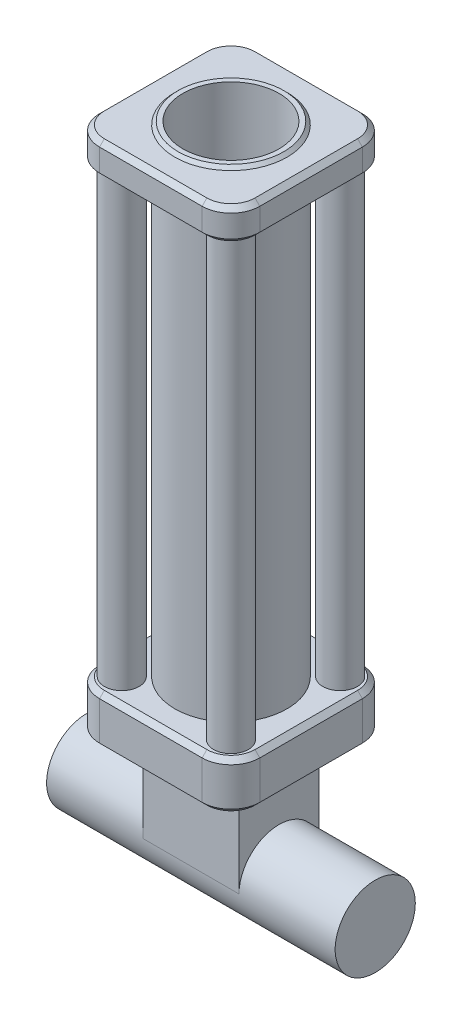
from build123d import *

# Parameters (mm, degrees)
SKETCH1_R                = 175
SKETCH1_R_2              = 150
BOSS_EXTRUDE1_DEPTH      = 1500
SKETCH2_W                = 500
SKETCH2_H                = 500
BOSS_EXTRUDE2_DEPTH      = 150
BOSS_EXTRUDE3_DEPTH      = 150
BOSS_EXTRUDE3_DEPTH_BACK = 150
BOSS_EXTRUDE4_DEPTH      = 450
BOSS_EXTRUDE4_DEPTH_BACK = 450
SKETCH4_R                = 125
CHAMFER2_SIZE            = 10
SKETCH5_W                = 500
SKETCH5_H                = 500
SKETCH5_R                = 154.887495166
BOSS_EXTRUDE5_DEPTH      = 100
BOSS_EXTRUDE6_REACH      = 1587.875
SKETCH6_R                = 54.226637303
CIRPATTERN1_COUNT        = 4
FILLET1_R                = 90
CHAMFER3_SIZE            = 15


with BuildPart() as part:
    # Sketch1 → Boss-Extrude1 (new body)
    with BuildSketch(Plane(origin=(0, 0, 0), x_dir=(1, 0, 0), z_dir=(0, 1, 0))):
        with Locations(Location((0, 0, 0), (0, 0, 270))):
            Circle(SKETCH1_R)
        with Locations(Location((0, 0, 0), (0, 0, 270))):
            Circle(SKETCH1_R_2, mode=Mode.SUBTRACT)
    extrude(amount=BOSS_EXTRUDE1_DEPTH)

    # Sketch2 → Boss-Extrude2 (add)
    with BuildSketch(Plane.XZ):
        Rectangle(SKETCH2_W, SKETCH2_H)
    extrude(amount=BOSS_EXTRUDE2_DEPTH)

    # Sketch3 → Boss-Extrude3 (add, two sides: drawn at the far end of the back side and taken through both)
    with BuildSketch(Plane(origin=(0, 0, 0), x_dir=(0, 0, -1), z_dir=(1, 0, 0)).offset(-BOSS_EXTRUDE3_DEPTH_BACK)):
        with BuildLine():
            Line((125, -150), (125, -450))
            ThreePointArc((125, -450), (0, -575), (-125, -450))
            Line((-125, -450), (-125, -150))
            Line((-125, -150), (125, -150))
        make_face()
    extrude(amount=BOSS_EXTRUDE3_DEPTH + BOSS_EXTRUDE3_DEPTH_BACK)

    # Sketch4 → Boss-Extrude4 (add, two sides: drawn at the far end of the back side and taken through both)
    with BuildSketch(Plane(origin=(0, 0, 0), x_dir=(0, 0, -1), z_dir=(1, 0, 0)).offset(-BOSS_EXTRUDE4_DEPTH_BACK)):
        with Locations((0, -450)):
            Circle(SKETCH4_R)
    extrude(amount=BOSS_EXTRUDE4_DEPTH + BOSS_EXTRUDE4_DEPTH_BACK)

    # Chamfer2
    chamfer2_edges = [part.edges().sort_by_distance(p)[0] for p in [
        (0, 1500, -175),
    ]]
    chamfer(chamfer2_edges, length=CHAMFER2_SIZE)

    # Sketch5 → Boss-Extrude5 (add)
    with BuildSketch(Plane(origin=(0, 1490, 0), x_dir=(1, 0, 0), z_dir=(0, 1, 0))):
        Rectangle(SKETCH5_W, SKETCH5_H)
        Circle(SKETCH5_R, mode=Mode.SUBTRACT)
    extrude(amount=-BOSS_EXTRUDE5_DEPTH)

    # Sketch6 → Boss-Extrude6 (add, up to next)
    with BuildSketch(Plane(origin=(0, 0, 0), x_dir=(1, 0, 0), z_dir=(0, 1, 0)), mode=Mode.PRIVATE) as boss_extrude6_sk1:
        with Locations(Location((-170.275340777, 170.275340777, 0), (0, 0, 90))):
            Circle(SKETCH6_R)
    boss_extrude6_tool1 = extrude(boss_extrude6_sk1.sketch, amount=BOSS_EXTRUDE6_REACH, mode=Mode.PRIVATE) - part.part
    boss_extrude6 = boss_extrude6_tool1.solids().sort_by_distance((-170.275341, 0, -170.275341))[0]
    add(boss_extrude6)

    # CirPattern1: Boss-Extrude6 ×4 about axis
    cirpattern1_axis = Axis((0, 0, 0), (0, 1, 0))
    for i in range(1, CIRPATTERN1_COUNT):
        add(boss_extrude6.rotate(cirpattern1_axis, i * 360 / CIRPATTERN1_COUNT))

    # Fillet1
    fillet1_edges = [part.edges().sort_by_distance(p)[0] for p in [
        (250, -75, -250),
        (250, -75, 250),
        (-250, -75, 250),
        (-250, -75, -250),
        (250, 1440, -250),
        (250, 1440, 250),
        (-250, 1440, 250),
        (-250, 1440, -250),
    ]]
    fillet(fillet1_edges, radius=FILLET1_R)

    # Chamfer3
    chamfer3_edges = [part.edges().sort_by_distance(p)[0] for p in [
        (250, -150, 0),
        (0, 0, -250),
        (-250, 0, 0),
        (0, 0, 250),
        (-223.639610307, 0, -223.639610307),
        (-223.639610307, 0, 223.639610307),
        (223.639610307, 0, 223.639610307),
        (223.639610307, 0, -223.639610307),
        (0, -150, -250),
        (0, -150, 250),
        (-250, -150, 0),
        (-223.639610307, -150, -223.639610307),
        (-223.639610307, -150, 223.639610307),
        (223.639610307, -150, 223.639610307),
        (223.639610307, -150, -223.639610307),
        (0, 1490, -250),
        (0, 1390, -250),
        (250, 1490, 0),
        (-250, 1490, 0),
        (0, 1490, 250),
        (223.639610307, 1490, -223.639610307),
        (223.639610307, 1490, 223.639610307),
        (-223.639610307, 1490, 223.639610307),
        (-223.639610307, 1490, -223.639610307),
        (-250, 1390, 0),
        (250, 1390, 0),
        (0, 1390, 250),
        (223.639610307, 1390, -223.639610307),
        (223.639610307, 1390, 223.639610307),
        (-223.639610307, 1390, 223.639610307),
        (-223.639610307, 1390, -223.639610307),
        (250, 0, 0),
    ]]
    chamfer(chamfer3_edges, length=CHAMFER3_SIZE)


solid = part.part
